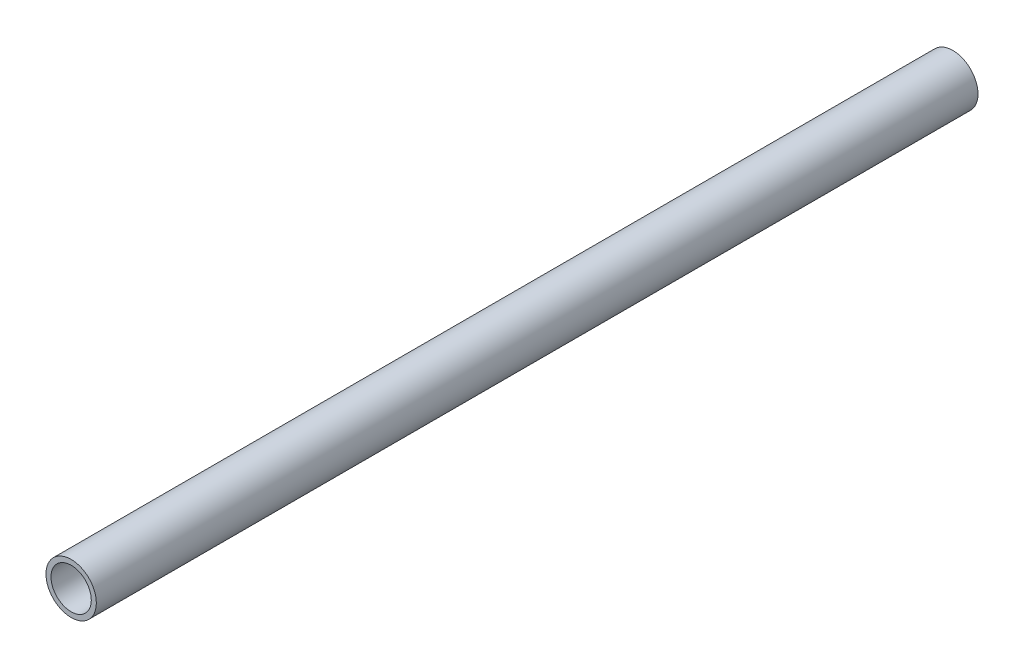
SolidWorks part; units mm, degrees
material "PP 共聚物"
ref_plane "前视基准面" through (0, 0, 0) normal (0, 0, 1) x (1, 0, 0)
ref_plane "上视基准面" through (0, 0, 0) normal (0, 1, 0) x (1, 0, 0)
ref_plane "右视基准面" through (0, 0, 0) normal (1, 0, 0) x (0, 0, -1)
sketch "草图1" plane through (0, 0, 0) normal (0, 0, 1) x (1, 0, 0)
  circle A0 centre (0, 0) radius 10
  dimension "D1" = 20
extrude "拉伸-薄壁1" add sketch "草图1" along normal blind 350 thin thin type one direction reverse wall 2
